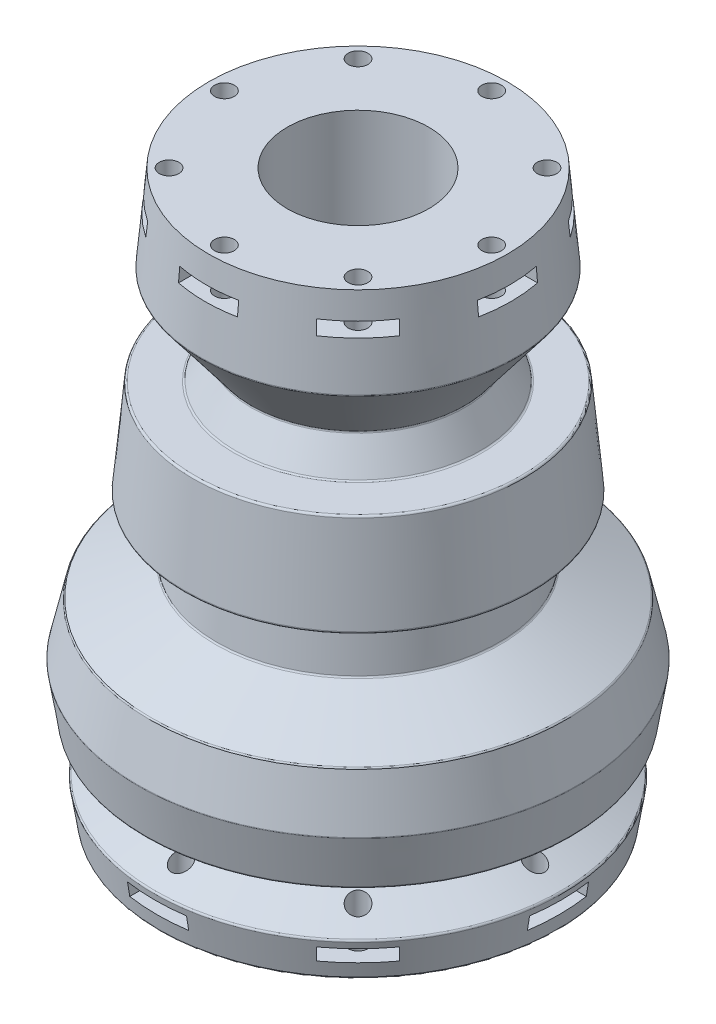
SolidWorks part; units mm, degrees
ref_plane "前视基准面" through (0, 0, 0) normal (0, 0, 1) x (1, 0, 0)
ref_plane "上视基准面" through (0, 0, 0) normal (0, 1, 0) x (1, 0, 0)
ref_plane "右视基准面" through (0, 0, 0) normal (1, 0, 0) x (0, 0, -1)
sketch "草图1" plane through (0, 0, 0) normal (0, 0, 1) x (1, 0, 0)
  line L0 (18, 0) -> (18, -143)
  line L1 (0, 0) -> (0, -140.0769) construction
  line L2 (18, -143) -> (50.5, -143)
  line L30 (50.5, -143) -> (52, -133.6)
  line L36 (52, -133.6) -> (37.3, -126.6)
  line L41 (37.3, -126.6) -> (38.5, -120.6)
  line L42 (38.5, -120.6) -> (54, -120.6)
  line L44 (54, -120.6) -> (56, -108.1)
  line L47 (56, -108.1) -> (53, -94.8)
  line L50 (53, -94.8) -> (36, -86.8)
  line L51 (36, -86.8) -> (34.5, -71.5)
  line L52 (34.5, -71.5) -> (44.3, -71.5)
  line L54 (44.3, -71.5) -> (42, -47)
  line L57 (42, -47) -> (31.3, -47)
  line L58 (31.3, -47) -> (27, -39)
  line L60 (27, -39) -> (40, -22)
  line L74 (40, -22) -> (38, 0)
  line L75 (38, 0) -> (40, -22)
  line L89 (40, -22) -> (27, -39)
  line L91 (27, -39) -> (31.3, -47)
  line L92 (31.3, -47) -> (42, -47)
  line L95 (42, -47) -> (44.3, -71.5)
  line L97 (44.3, -71.5) -> (34.5, -71.5)
  line L98 (34.5, -71.5) -> (36, -86.8)
  line L99 (36, -86.8) -> (53, -94.8)
  line L101 (53, -94.8) -> (56, -108.1)
  line L104 (56, -108.1) -> (54, -120.6)
  line L106 (54, -120.6) -> (38.5, -120.6)
  line L107 (38.5, -120.6) -> (37.3, -126.6)
  line L112 (37.3, -126.6) -> (52, -133.6)
  line L118 (52, -133.6) -> (50.5, -143)
  line L132 (38, 0) -> (0, 0)
  dimension "D1" = 22
  dimension "D2" = 38
  dimension "D3" = 40
  dimension "D4" = 17
  dimension "D5" = 27
  dimension "D6" = 8
  dimension "D7" = 31.3
  dimension "D8" = 42
  dimension "D9" = 24.5
  dimension "D10" = 44.3
  dimension "D11" = 34.5
  dimension "D12" = 15.3
  dimension "D13" = 36
  dimension "D14" = 8
  dimension "D15" = 53
  dimension "D16" = 13.3
  dimension "D17" = 56
  dimension "D18" = 12.5
  dimension "D19" = 38.5
  dimension "D20" = 54
  dimension "D21" = 6
  dimension "D22" = 37.3
  dimension "D23" = 18
  dimension "D24" = 7
  dimension "D25" = 32.5
  dimension "D26" = 143
  dimension "D27" = 52
revolve "旋转1" add sketch "草图1" angle 360 about L1
sketch "草图2" plane through (0, 0, 0) normal (0, 1, 0) x (1, 0, 0)
  line L0 (0, 0) -> (0, -38) construction
  line L1 (7.5, -51) -> (-7.5, -51)
  line L2 (7.5, -51) -> (7.5, -25)
  line L3 (7.5, -25) -> (-7.5, -25)
  line L4 (-7.5, -51) -> (-7.5, -25)
  line L5 (7.5, -51) -> (-7.5, -25) construction
  line L6 (7.5, -25) -> (-7.5, -51) construction
  circle A0 centre (0, 0) radius 38 construction
  dimension "D1" = 15
  dimension "D2" = 13
extrude "切除-拉伸1" cut sketch "草图2" along normal blind 3.5 from offset 10 offset against normal yes
sketch "草图3" plane through (0, 0, 0) normal (0, 1, 0) x (1, 0, 0)
  line L0 (0, 0) -> (0, -34) construction
  line L1 (0, -34) -> (0, -38) construction
  circle A0 centre (0, 0) radius 38 construction
  circle A1 centre (0, -34) radius 2.5
  dimension "D2" = 5
  dimension "D1" = 4
extrude "切除-拉伸2" cut sketch "草图3" against normal blind 15
sketch "草图4" plane through (0, -143, 0) normal (0, -1, 0) x (1, 0, 0)
  line L0 (0, 45) -> (0, 0) construction
  circle A0 centre (0, 45) radius 2.5
  dimension "D1" = 5
  dimension "D2" = 45
extrude "切除-拉伸3" cut sketch "草图4" against normal blind 15
sketch "草图5" plane through (0, -143, 0) normal (0, -1, 0) x (1, 0, 0)
  line L1 (7.5, 35) -> (-7.5, 35)
  line L2 (7.5, 35) -> (7.5, 55)
  line L3 (7.5, 55) -> (-7.5, 55)
  line L4 (-7.5, 35) -> (-7.5, 55)
  line L5 (7.5, 35) -> (-7.5, 55) construction
  line L6 (7.5, 55) -> (-7.5, 35) construction
  point P0 (0, 45)
  dimension "D1" = 15
  dimension "D2" = 20
extrude "切除-拉伸4" cut sketch "草图5" against normal blind 3.5 from offset 4 offset against normal yes
pattern_circular "阵列(圆周)1" count 8 over 360 about axis through (0, 0, 0) along (0, 1, 0) of "切除-拉伸1", "切除-拉伸2", "切除-拉伸4", "切除-拉伸3"
sketch "草图6" plane through (0, -143, 0) normal (0, -1, 0) x (1, 0, 0)
  circle A0 centre (0, 0) radius 18
  circle A1 centre (0, 0) radius 25
  circle A2 centre (0, 0) radius 18 construction
  dimension "D1" = 50
extrude "凸台-拉伸1" add sketch "草图6" along normal blind 15
sketch "草图7" plane through (0, 0, 0) normal (0, 0, 1) x (1, 0, 0)
  line L0 (0, -151) -> (0, -158) construction
  line L1 (-25, -158) -> (25, -158) construction
  circle A0 centre (0, -151) radius 2.75
  dimension "D1" = 5.5
  dimension "D2" = 7
extrude "切除-拉伸5" cut sketch "草图7" against normal blind 50
sketch "草图8" plane through (0, 0, 0) normal (0, 0, 1) x (1, 0, 0)
  circle A0 centre (0, -151) radius 5
  dimension "D1" = 10
extrude "切除-拉伸6" cut sketch "草图8" against normal blind 50 from offset 24 offset against normal yes
pattern_circular "阵列(圆周)2" count 4 over 360 about axis through (0, 0, 0) along (0, 1, 0) of "切除-拉伸6", "切除-拉伸5"
fillet "圆角1" radius 0.5 15 edges at (0, -22, 40) (0, -39, 27) (0, -47, 31.3) (0, -47, 42) (0, -71.5, 44.3) (0, -71.5, 34.5) (0, -86.8, 36) (0, -94.8, 53) (0, -108.1, 56) (0, -120.6, 54) (0, -120.6, 38.5) (0, -126.6, 37.3) (0, -133.6, 52) (0, -143, 50.5) (0, -143, 25)
